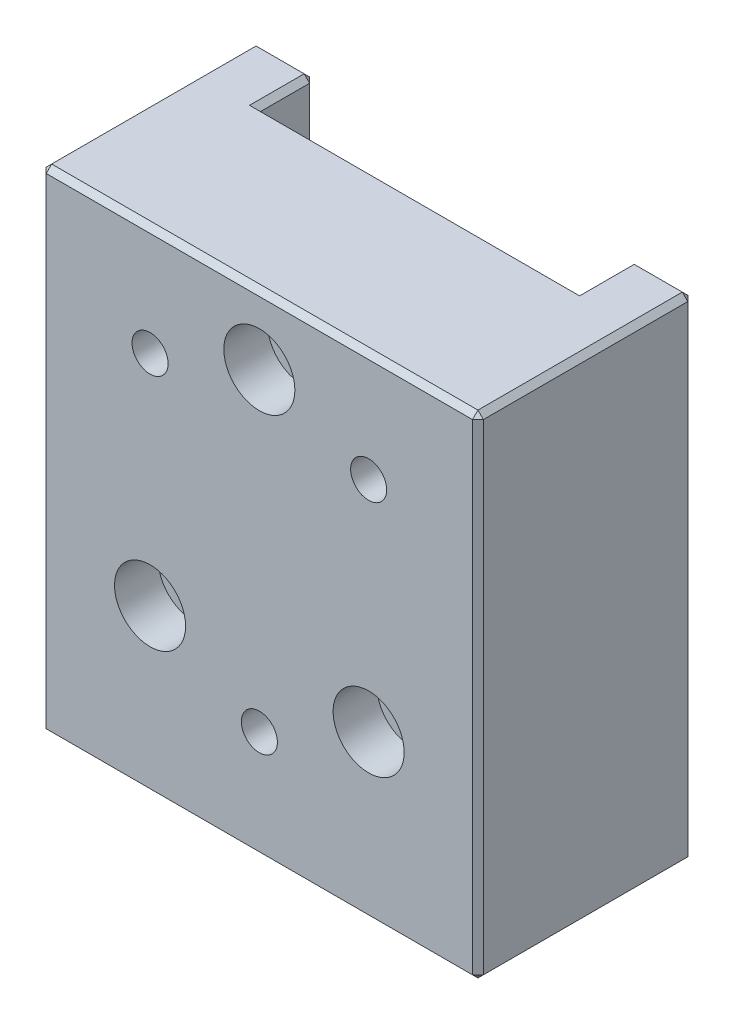
from build123d import *

# Parameters (mm, degrees)
SKETCH_1_W                   = 40
SKETCH_1_H                   = 45
EXTRUDE_1_DEPTH              = 7.35
HOLE_WIZARD_M3_1_D           = 3.4
HOLE_WIZARD_M3_1_CBORE_D     = 6.5
HOLE_WIZARD_M3_1_CBORE_DEPTH = 4
SKETCH_5_W                   = 5.4
SKETCH_5_H                   = 45
EXTRUDE_2_DEPTH              = 5
HOLE_WIZARD_M4_2_D           = 3.3
CHAMFER_1_SIZE               = 0.5


with BuildPart() as part:
    # 草图1 → 凸台-拉伸1 (new, symmetric)
    with BuildSketch(Plane.XY):
        Rectangle(SKETCH_1_W, SKETCH_1_H)
    extrude(amount=EXTRUDE_1_DEPTH, both=True)

    # M3 六角凹头螺钉的柱形沉头孔1 (through all)
    with Locations(Plane.XY.offset(7.35)):
        with Locations((0, 16.2), (-10, -7.5), (10, -7.5)):
            CounterBoreHole(HOLE_WIZARD_M3_1_D / 2, HOLE_WIZARD_M3_1_CBORE_D / 2, HOLE_WIZARD_M3_1_CBORE_DEPTH)

    # 草图5 → 凸台-拉伸2 (add)
    with BuildSketch(Plane(origin=(0, 0, -7.35), x_dir=(-1, 0, 0), z_dir=(0, 0, -1))):
        with Locations((-17.3, 0)):
            Rectangle(SKETCH_5_W, SKETCH_5_H)
        with Locations((17.3, 0)):
            Rectangle(SKETCH_5_W, SKETCH_5_H)
    extrude(amount=EXTRUDE_2_DEPTH)

    # M4 螺纹孔2 (through all)
    with Locations(Plane.XY.offset(7.35)):
        with Locations((10, 12.5), (-10, 12.5), (0, -12.5)):
            Hole(HOLE_WIZARD_M4_2_D / 2)

    # 倒角1
    chamfer_1_edges = [part.edges().sort_by_distance(p)[0] for p in [
        (-20, 0, 7.35),
        (0, -22.5, 7.35),
        (0, 22.5, -7.35),
        (14.6, -22.5, -9.85),
        (14.6, 22.5, -9.85),
        (20, 0, -12.35),
        (17.3, -22.5, -12.35),
        (14.6, 0, -12.35),
        (17.3, 22.5, -12.35),
        (20, 0, 7.35),
        (0, -22.5, -7.35),
        (-14.6, 22.5, -9.85),
        (-14.6, -22.5, -9.85),
        (-14.6, 0, -12.35),
        (-17.3, -22.5, -12.35),
        (-20, 0, -12.35),
        (-17.3, 22.5, -12.35),
        (0, 22.5, 7.35),
        (20, -22.5, -2.5),
        (-20, -22.5, -2.5),
        (-20, 22.5, -2.5),
        (20, 22.5, -2.5),
    ]]
    chamfer(chamfer_1_edges, length=CHAMFER_1_SIZE)


solid = part.part
